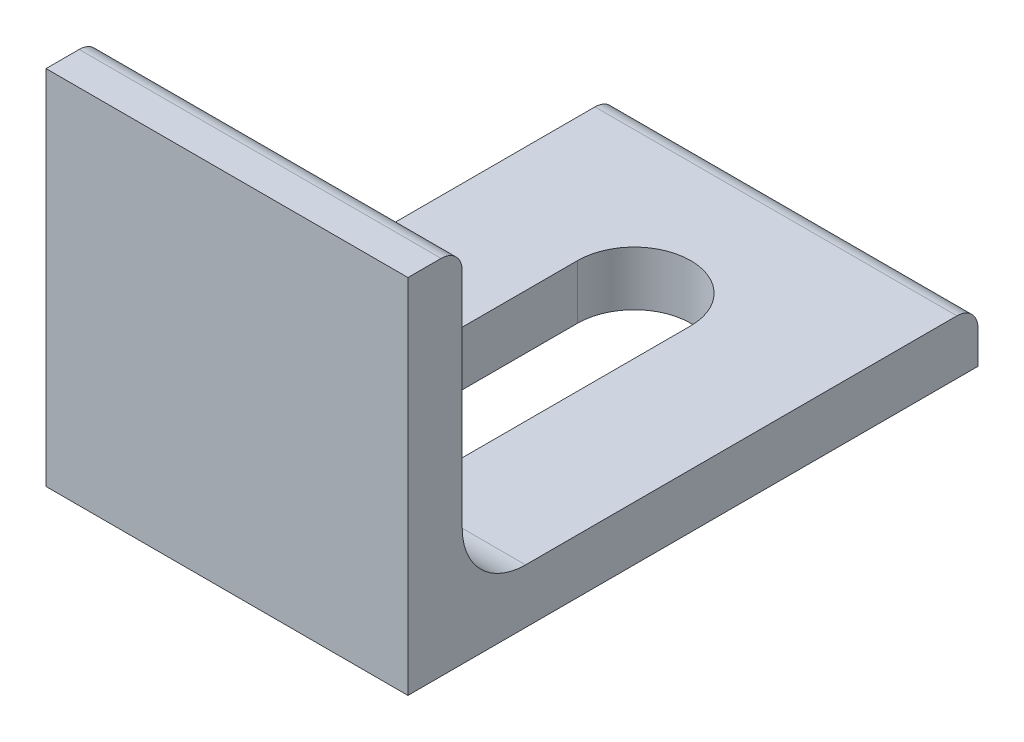
SolidWorks part; units mm, degrees
material "普通碳钢"
ref_plane "Front Plane" through (0, 0, 0) normal (0, 0, 1) x (1, 0, 0)
ref_plane "Top Plane" through (0, 0, 0) normal (0, 1, 0) x (1, 0, 0)
ref_plane "Right Plane" through (0, 0, 0) normal (1, 0, 0) x (0, 0, -1)
sketch3d "3DSketch1"
  line L0 (220, 114, 0) -> (180, 114, 0)
  line L1 (245, 114, 0) -> (285, 114, 0) construction
  dimension "D1" = 40
other "Hot-rolled unequal angle GB∕T 706-2008 63 X 40 X 6 (1)"
ref_plane "Plane1" through (220, 114, 0) normal (-1, 0, 0) x (0, 1, 0)
sketch "Sketch1" plane through (220, 114, 0) normal (-1, 0, 0) x (0, 1, 0)
  line L0 (0, 0) -> (0, 63)
  line L1 (0, 31.5) -> (6, 31.5) construction
  line L2 (6, 60.6667) -> (6, 13)
  line L3 (13, 6) -> (37.6667, 6)
  line L4 (20, 6) -> (20, 0) construction
  line L5 (40, 0) -> (0, 0)
  line L6 (0, 63) -> (3.6667, 63)
  line L7 (40, 0) -> (40, 3.6667)
  arc A0 (40, 3.6667) -> (37.6667, 6) centre (37.6667, 3.6667) ccw
  arc A1 (3.6667, 63) -> (6, 60.6667) centre (3.6667, 60.6667) cw
  arc A2 (13, 6) -> (6, 13) centre (13, 13) cw
  point P10 (20, 0)
  point P14 (0, 31.5)
  point P15 (6, 31.5)
  point P16 (20, 6)
  point P21 (0, 0)
sketch "Sketch2" plane through (0, 120, 0) normal (0, 1, 0) x (1, 0, 0)
  line L0 (200, 45) -> (200, 20) construction
  line L1 (206.25, 45) -> (206.25, 20)
  line L2 (193.75, 45) -> (193.75, 20)
  line L3 (180, 13) -> (180, 60.6667) construction
  line L4 (220, 0) -> (180, 0) construction
  arc A0 (206.25, 45) -> (193.75, 45) centre (200, 45) ccw
  arc A1 (193.75, 20) -> (206.25, 20) centre (200, 20) ccw
  point P2 (200, 32.5)
  dimension "D1" = 12.5
  dimension "D2" = 25
  dimension "D3" = 20
  dimension "D4" = 20
extrude "Cut-Extrude1" cut sketch "Sketch2" against normal blind 10
equation "\"D2@Sketch1\" = \"Radius_1@Sketch1\" / 3"
equation "\"D4@Sketch1\" = \"D1@Sketch1\""
